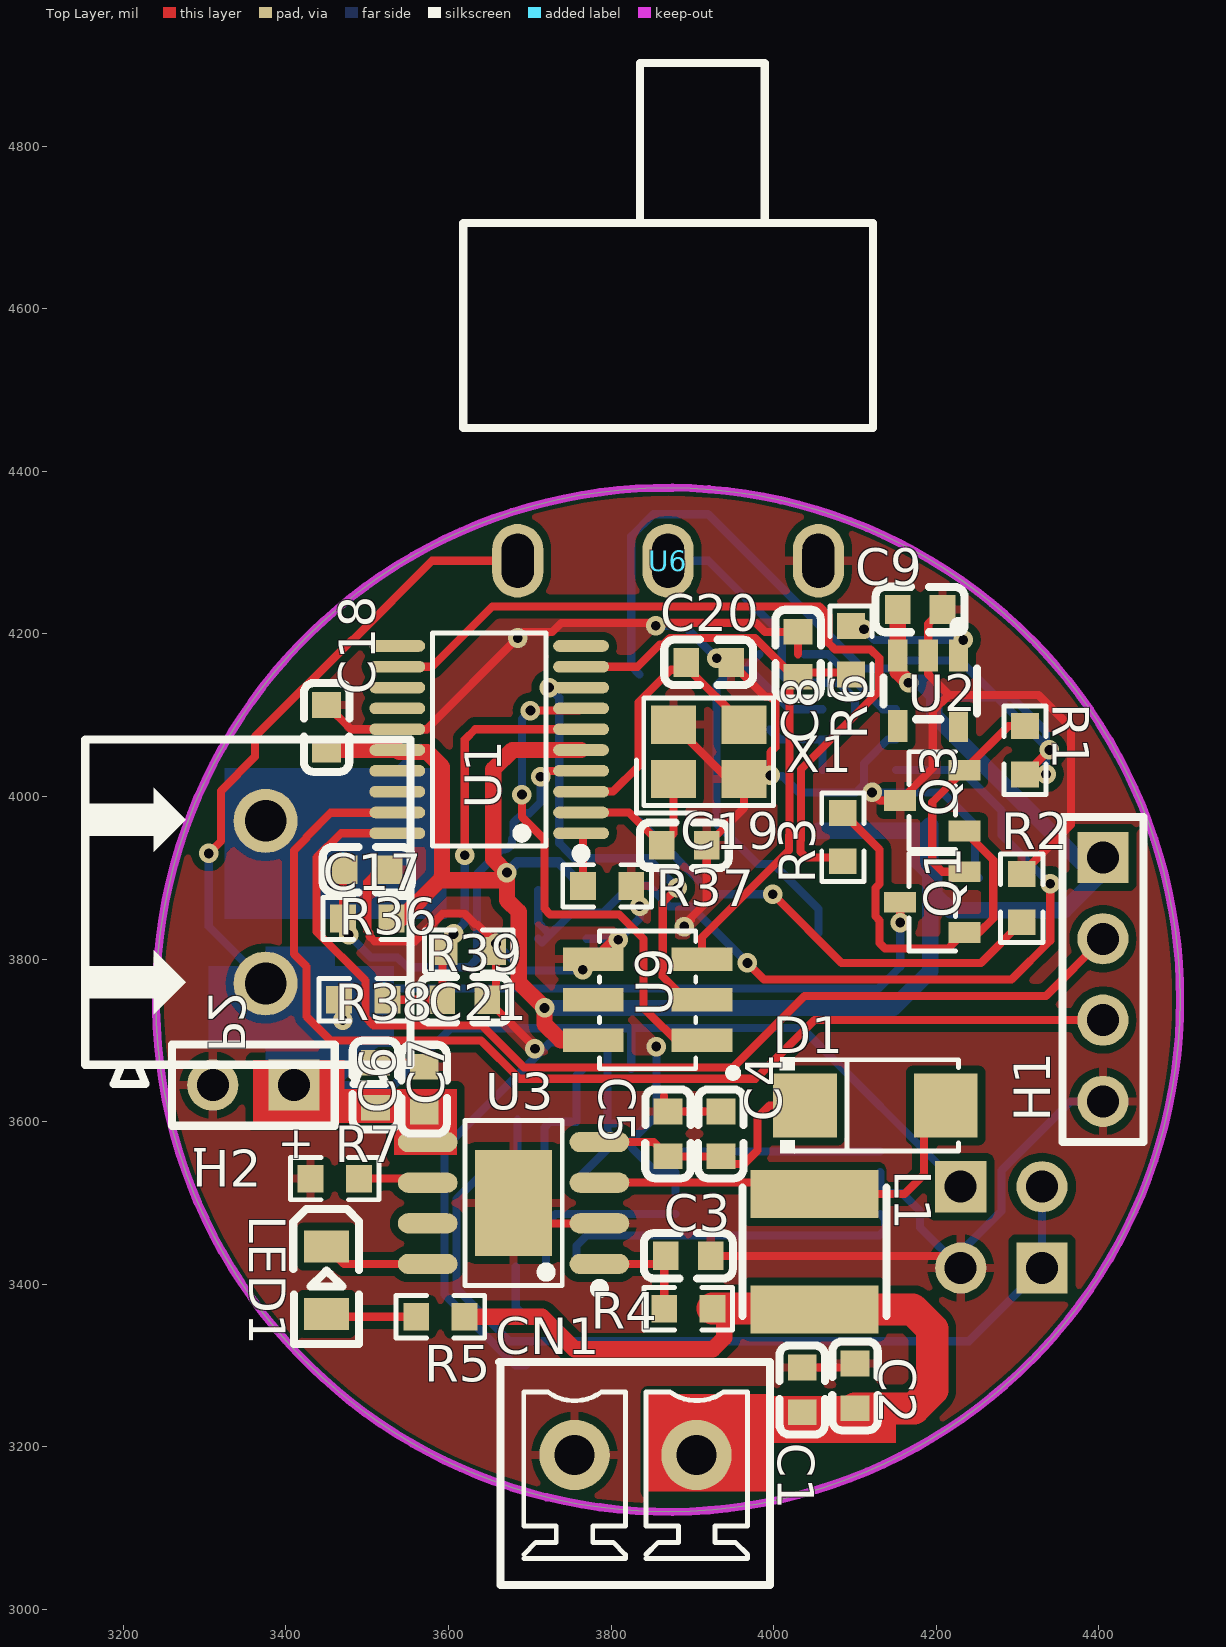
[diagram p0: Top Layer view]
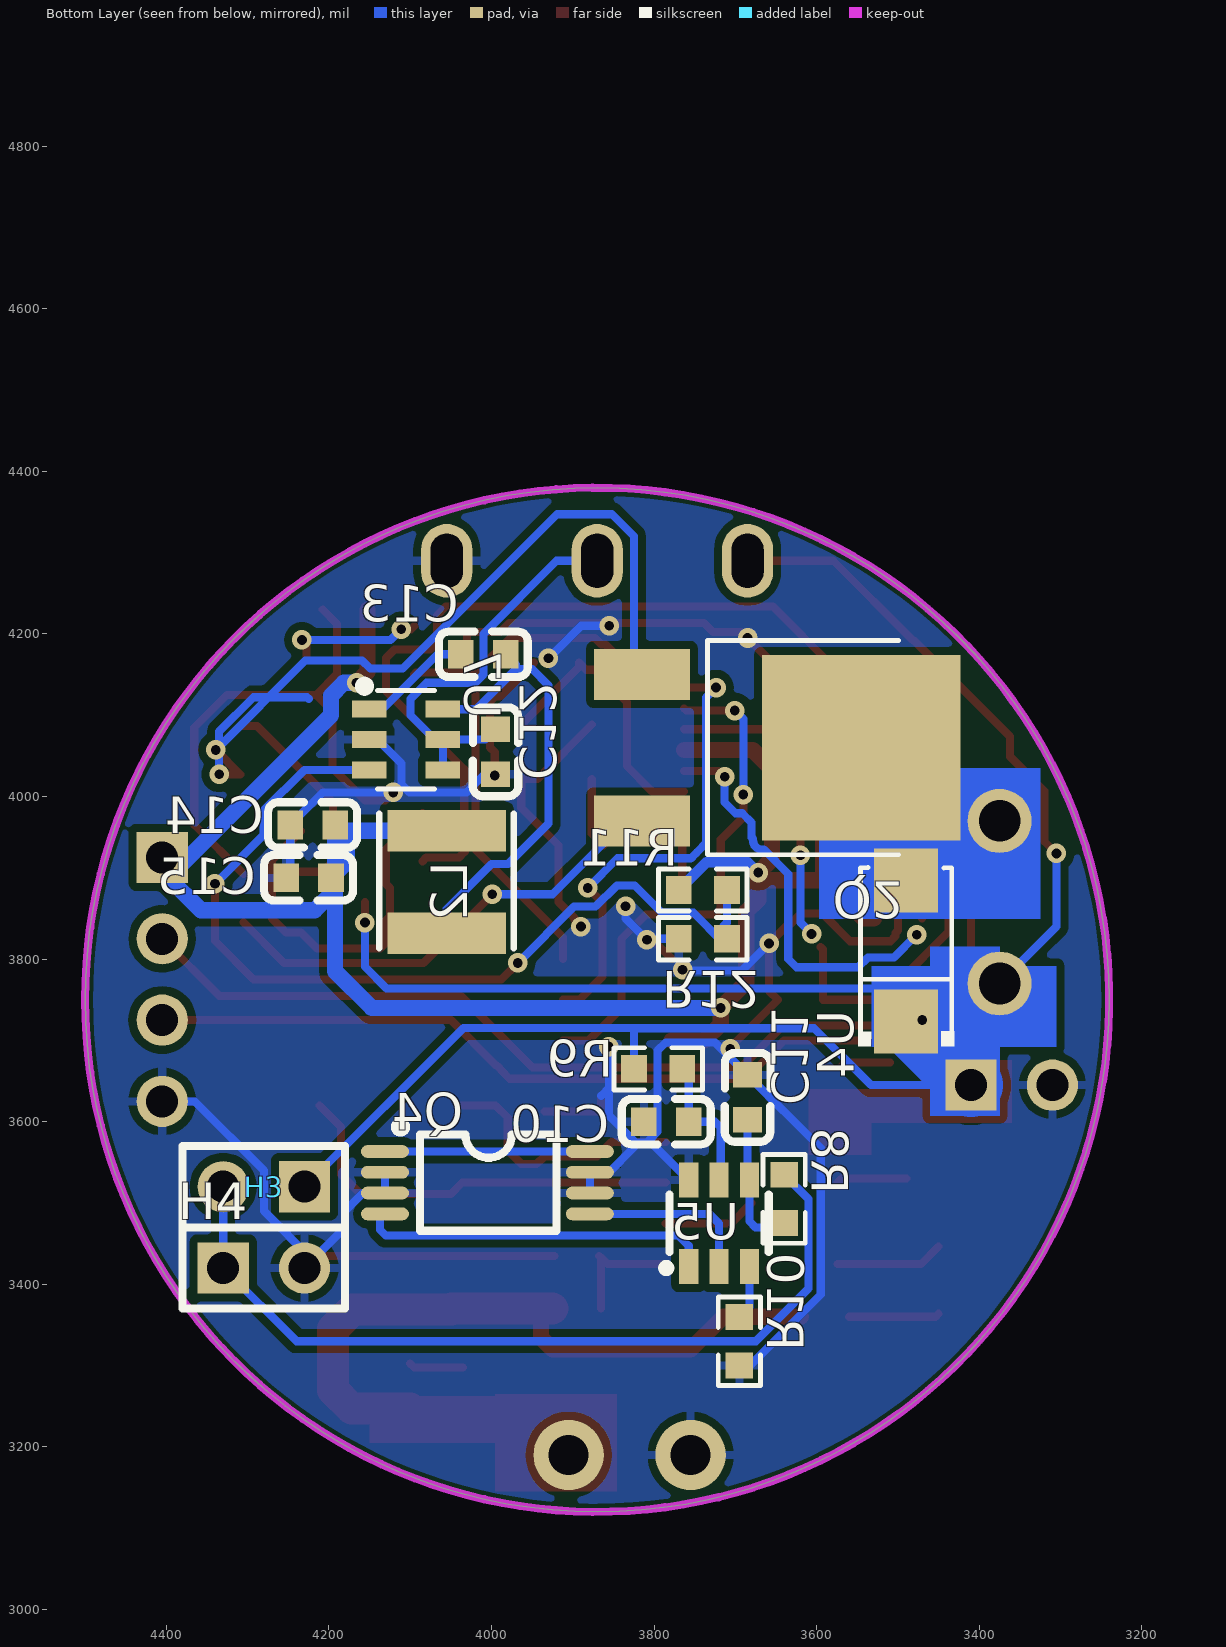
[diagram p1: Bottom Layer view, seen from below]
# Altium PCB MISC80546.pcbdoc
Units mil, origin at the board's own origin, x right, y up, seen from the top; angles counter-clockwise.
Board outline 1259.8 x 1259.8 mil, 2 copper layers (Top Layer, Bottom Layer), stack 62.2 mil thick; 59 components, 40 nets, 172 pads, 33 vias.

## Layer stack, top to bottom
Top Solder Mask Layer: solder mask 0.4, Dk 3.3
Top Layer: signal copper 1.4
Dielectric1: surface 59.4, FR4, Dk 4.5
Bottom Layer: signal copper 1.4
Bottom Solder Mask Layer: solder mask 0.4, Dk 3.3

## Board outline
4499.9,3750 ccw(c3870,3750) 3240.1,3750 ccw(c3870,3750)

## Design rules (kind name [scope] priority, off if disabled: settings)
BoardOutlineClearance copperThickness1oz [All] p0: genericclearance=10 ignorepadtopadclearanceinfootprint=FALSE except(0: Arc-SplitContinuation Track-SplitContinuation SMDPad-SplitContinuation THPad-SplitContinuation Via-SplitContinuation Fill-SplitContinuation Poly-SplitContinuation Region-SplitContinuation Text-SplitContinuation)
BoardOutlineClearance copperThickness2oz [All] p0: genericclearance=10 ignorepadtopadclearanceinfootprint=FALSE except(0: Arc-SplitContinuation Track-SplitContinuation SMDPad-SplitContinuation THPad-SplitContinuation Via-SplitContinuation Fill-SplitContinuation Poly-SplitContinuation Region-SplitContinuation Text-SplitContinuation)
BoardOutlineClearance otherClearance [All] p0: genericclearance=10 ignorepadtopadclearanceinfootprint=FALSE except(0: Arc-SplitContinuation Track-SplitContinuation SMDPad-SplitContinuation THPad-SplitContinuation Via-SplitContinuation Fill-SplitContinuation Poly-SplitContinuation Region-SplitContinuation Text-SplitContinuation)
Clearance copperThickness1oz [All] p1: gap=7 ignorepadtopadclearanceinfootprint=FALSE
Clearance copperThickness2oz [All] p1: gap=7 ignorepadtopadclearanceinfootprint=FALSE
Clearance otherClearance [All] p1: gap=7 ignorepadtopadclearanceinfootprint=FALSE
DiffPairsRouting differentialPair [All] p1: maxuncoupledlength=10 minlimit=6 maxlimit=Infinity mostfreqgap=6 toplayer_minwidth=5 toplayer_prefwidth=10 toplayer_maxwidth=100 bottomlayer_minwidth=5 bottomlayer_prefwidth=10 bottomlayer_maxwidth=100
PasteMaskExpansion pasteMaskExpansion [All] p1: expansion=0
PlaneConnect innerPlane [All] p1: planeconnectstyle=Relief reliefexpansion=20 reliefentries=4 reliefconductorwidth=10 reliefairgap=10
PolygonConnect copperRegion [All] p1: connectstyle=Relief reliefentries=4 reliefconductorwidth=10 polygonreliefangle="90 Angle" airgapwidth=10
RoutingVias viaSize [All] p1: viastyle="Through Hole" holewidth=12.0078 minholewidth=11.811 maxholewidth=248.0314 width=12.0078 minwidth=11.811 maxwidth=248.0314
SolderMaskExpansion solderMaskExpansion [IsVia] p1: useseparateexpansions=TRUE expansion=-1000 expansionbottom=-1000
SolderMaskExpansion solderMaskExpansion [All] p2: useseparateexpansions=TRUE expansion=2 expansionbottom=2
Width copperThickness1oz [All] p1: maxlimit=100 minlimit=5 preferedwidth=10
Width copperThickness2oz [All] p1: maxlimit=100 minlimit=8 preferedwidth=20

## Components (designator, comment, footprint, x,y, rotation, side; value= is the part's Value field where it differs from the comment)
C1 "100nF" C0603 4035,3270 r270 top
C2 "100nF" C0603 4100,3275 r270 top
C3 "100nF" C0603 3895,3435 r180 top
C4 "100nF" C0603 3935,3585 r90 top
C5 "100nF" C0603 3870,3585 r270 top
C6 "100nF" C0603 3510,3645 r90 top
C7 "100nF" C0603 3570,3640 r90 top
C8 "100nF" C0603 4030,4175 r270 top
C9 "100nF" C0603 4180,4230 r0 top
C10 "100nF" C0603 3785,3600 r180 bottom
C11 "100nF" C0603 3685,3630 r90 bottom
C12 "100nF" C0603 3995,4055 r90 bottom
C13 "100nF" C0603 4010,4175 r0 bottom
C14 "100nF" C0603 4220,3965 r180 bottom
C15 "100nF" C0603 4225,3900 r180 bottom
C17 "100nF" C0603 3500,3910 r0 top
C18 "100nF" C0603 3450,4085 r90 top
C19 "100nF" C0603 3890,3940 r0 top
C20 "100nF" C0603 3920,4165 r0 top
C21 "100nF" C0603 3620,3750 r0 top
CN1 "WJ15EDGVC-3.81-02P-14-00A" CONN-TH_WJ15EDGVC-3.81-2P 3830,3190 r0 top
D1 "SS34" SMA_L4.3-W2.6-LS5.2-RD 4125,3620 r0 top
H1 "LAIL-PZ2.54-4P-L" CONN-TH_LAIL-PZ2.54-4P-L 4405,3775 r270 top
H2 "LAIL-PZ2.54-2P-L" CONN-TH_LAIL-PZ2.54-2P-L 3360,3645 r180 top
H3 "LAIL-PZ2.54-2P-L" CONN-TH_LAIL-PZ2.54-2P-L 4280,3520 r0 bottom
H4 "LAIL-PZ2.54-2P-L" CONN-TH_LAIL-PZ2.54-2P-L 4280,3420 r180 bottom
L1 "2.2uH" IND-SMD_L4.0-W4.0_LQH44PN2R2MP0L 4050,3440 r270 top
L2 "4.7uH" IND-SMD_L4.0-W4.0_SMNR4012 4055,3895 r90 bottom
LED1 "KT-0805W" LED0805-R-RD 3450,3405 r270 top
P2 "WJ500V-5.08-2P" CONN-TH_2P-P5.00_WJ500V-5.08-2P 3375,3870 r90 top
Q1 "SS8050(RANGE:200-350)" SOT-23-3_L2.9-W1.3-P1.90-LS2.4-BR 4195,3870 r0 top
Q2 "CMD075N06L" TO-252-2_L6.6-W6.1-P4.57-LS9.9-BR-CW 3680,4060 r0 bottom
Q3 "SS8550 Y2(RANGE:200-350)" SOT-23-3_L2.9-W1.3-P1.90-LS2.4-BR 4195,3995 r0 top
Q4 "AP8205A" TSSOP-8_L4.4-W3.0-P0.65-LS6.4-BL-2 4005,3525 r270 bottom
R1 "10K" R0603 4309.1,4057 r270 top
R2 "10K" R0603 4305,3875 r270 top
R3 "10K" R0603 4085,3950 r90 top
R4 "10K" R0603 3895,3370 r0 top
R5 "10K" R0603 3590,3360 r0 top
R6 "10K" R0603 4095,4180 r90 top
R7 "10K" R0603 3460,3530 r180 top
R8 "10K" R0603 3640,3505 r270 bottom
R9 "10K" R0603 3795,3665 r180 bottom
R10 "10K" R0603 3695,3330 r270 bottom
R11 "10K" R0603 3740,3885 r180 bottom
R12 "10K" R0603 3740,3825 r0 bottom
R36 "10K" R0603 3500,3850 r0 top
R37 "10K" R0603 3795,3890 r0 top
R38 "10K" R0603 3495,3750 r180 top
R39 "10K" R0603 3625,3810 r180 top
U1 "GD32E230F8P6TR" TSSOP-20_L6.5-W4.4-P0.65-LS6.4-BL 3650,4070 r90 top
U2 "SC01T" SOT-23-5_L2.9-W1.6-P0.95-LS2.8-BR 4190,4130 r90 top
U3 "PW4584A" ESOP-8_L4.9-W3.9-P1.27-LS6.0-BL-EP-1 3680,3500 r90 top
U4 "SS36" SMA_L4.3-W2.6-LS5.1-RD 3490,3810 r90 bottom
U5 "HY2120-CB" SOT-23-6_L2.9-W1.6-P0.95-LS2.8-BR 3720,3475 r270 bottom
U6 "SS-12D06G5R" SW-TH_SS-12D06G5R 3870,4290 r180 top
U7 "MT2492" SOT-23-6_L2.9-W1.6-P0.95-LS2.8-BL_3 4105,4070 r270 bottom
U9 "LAIL-PM1.27-3PX2-T" HDR-SMD_6P-P1.27_LAIL-PM1.27-3PX2-T 3845,3750 r90 top locked
X1 "8MHz" CRYSTAL-SMD_4P-L3.2-W2.5-BL 3920,4055 r0 top

## Footprints (in the part's own frame and the unit in brackets; to place one, negate y for a bottom-side part, rotate by r counter-clockwise, add the part's x,y. Pads: shape width x height; smd on the part's side, far side on the other; paste and mask are expansions set on the pad)
C0603 [mil]
  rect 31.5x35.4 smd: 1(-27.6,0) 2(27.6,0)
  silkscreen extent -55,-28 55,28
CONN-TH_2P-P5.00_WJ500V-5.08-2P [mil]
  round 78.7 hole 51.2: 1(-100,0) 2(100,0)
  silkscreen extent -224,-178 200,222
CONN-TH_LAIL-PZ2.54-2P-L [mil]
  rect 63x63 hole 39.4 paste+0 mask+2: 1(-50,0)
  round 63 hole 39.4 paste+0 mask+2: 2(50,0)
  silkscreen extent -100,-50 100,50
CONN-TH_LAIL-PZ2.54-4P-L [mil]
  rect 63x63 hole 39.4 paste+0 mask+2: 1(-150,0)
  round 63 hole 39.4 paste+0 mask+2: 2(-50,0) 3(50,0) 4(150,0)
  silkscreen extent -200,-50 200,50
CONN-TH_WJ15EDGVC-3.81-2P [mil]
  round 86.6 hole 49.2: 1(-75,0) 2(75,0)
  silkscreen extent -168,-160 165,114
CRYSTAL-SMD_4P-L3.2-W2.5-BL [mil]
  rect 55.1x47.2 smd: 1(-43.3,-33.5) 2(43.3,-33.5) 3(43.3,33.5) 4(-43.3,33.5)
  silkscreen extent -89,-75 80,66
ESOP-8_L4.9-W3.9-P1.27-LS6.0-BL-EP-1 [mil]
  oval 24.8x73.4 smd: 1(-75,-105.6) 2(-25,-105.6) 3(25,-105.6) 4(75,-105.6) 5(75,105.6) 6(25,105.6) 7(-25,105.6) 8(-75,105.6)
  rect 129.9x94.5 smd paste+0 mask+2: 9(0,0)
  silkscreen extent -111,-111 101,60
HDR-SMD_6P-P1.27_LAIL-PM1.27-3PX2-T [mil]
  rect 29.1x74.8 smd paste+0 mask+2: 1(-50,-66.9) 2(-50,66.9) 3(0,-66.9) 4(0,66.9) 5(50,-66.9) 6(50,66.9)
  silkscreen extent -95,-110 85,59
IND-SMD_L4.0-W4.0_LQH44PN2R2MP0L [mil]
  rect 59.1x157.5 smd: 1(-70.9,0) 2(70.9,0)
  silkscreen extent -79,-89 79,89
IND-SMD_L4.0-W4.0_SMNR4012 [mil]
  rect 51.2x145.7 smd: 1(-63,0) 2(63,0)
  silkscreen extent -82,-82 84,83
LED0805-R-RD [mil]
  rect 39.4x55.1 smd: 1(41.3,0) 2(-41.3,0)
  silkscreen extent -88,-41 78,40
R0603 [mil]
  rect 31.8x34 smd paste-3937 mask+2: 1(-29.7,0) 2(29.7,0)
  silkscreen extent -55,-26 55,26
SMA_L4.3-W2.6-LS5.1-RD [mil]
  rect 78.7x78.7 smd: 1(-86.6,0) 2(86.6,0)
  silkscreen extent -117,-59 102,59
SMA_L4.3-W2.6-LS5.2-RD [mil]
  rect 78.7x78.7 smd: 1(-86.6,0) 2(86.6,0)
  silkscreen extent -117,-59 102,59
SOT-23-3_L2.9-W1.3-P1.90-LS2.4-BR [mil]
  rect 39.4x25.6 smd: 1(39.4,-37.4) 2(39.4,37.4) 3(-39.4,0)
  silkscreen extent -29,-60 29,60
SOT-23-5_L2.9-W1.6-P0.95-LS2.8-BR [mil]
  rect 39.4x23.6 smd paste+0 mask+2: 1(43.3,-37.4) 2(43.3,0) 3(43.3,37.4) 4(-43.3,37.4) 5(-43.3,-37.4)
  silkscreen extent -35,-60 85,55
SOT-23-6_L2.9-W1.6-P0.95-LS2.8-BL_3 [mil]
  rect 20.9x42.2 smd: 1(-37.4,-45.2) 2(0,-45.2) 3(37.4,-45.2) 4(37.4,45.2) 5(0,45.2) 6(-37.4,45.2)
  silkscreen extent -72,-57 61,35
SOT-23-6_L2.9-W1.6-P0.95-LS2.8-BR [mil]
  rect 43.3x23.6 smd paste+0 mask+2: 1(53.2,-37.4) 2(53.2,0) 3(53.2,37.4) 4(-53.2,37.4) 5(-53.2,0) 6(-53.2,-37.4)
  silkscreen extent -35,-70 60,61
SW-TH_SS-12D06G5R [mil]
  oval 63x90.6 hole 39.4 slot 66.9 at 90 deg: 1(-185,0) 2(0,0) 3(185,0)
  silkscreen extent -252,-612 252,-163
TO-252-2_L6.6-W6.1-P4.57-LS9.9-BR-CW [mil]
  rect 118.1x63 smd: 1(134.8,-90.2) 3(134.8,90.2)
  rect 244.1x228.3 smd: 2(-134.8,0)
  silkscreen extent -180,-132 54,132
TSSOP-8_L4.4-W3.0-P0.65-LS6.4-BL-2 [mil]
  oval 15.7x59.1 smd: 1(-38.4,-126) 2(-12.8,-126) 3(12.8,-126) 4(38.4,-126) 5(38.4,126) 6(12.8,126) 7(-12.8,126) 8(-38.4,126)
  silkscreen extent -74,-113 59,85
TSSOP-20_L6.5-W4.4-P0.65-LS6.4-BL [mil]
  oval 14.3x68.6 smd: 1(-115.2,-113) 2(-89.6,-113) 3(-64,-113) 4(-38.4,-113) 5(-12.8,-113) 6(12.8,-113) 7(38.4,-113) 8(64,-113) 9(89.6,-113) 10(115.2,-113) 11(115.2,113) 12(89.6,113) 13(64,113) 14(38.4,113) 15(12.8,113) 16(-12.8,113) 17(-38.4,113) 18(-64,113) 19(-89.6,113) 20(-115.2,113)
  silkscreen extent -146,-119 131,70

## Via types
v1: diameter 24, hole 12, Top Layer to Bottom Layer, 33 vias

## Nets (pads, with @x,y where several pads share a name; then routed paths per layer and width w, separated by ;. In a path a pad name is that pad's centre, name@x,y a point inside that pad or via, vN(x,y) a via of type N, cw(c..) or ccw(c..) an arc to the next point about the centre after c; other vN are vias at no path point)
$1N2: Q1.1 Q3.1 R3.2 | length 463.1
  Top Layer w10: R3.2 4130,3934.7 4130,3892.4 4125,3887.3 4125,3852.7 4130,3847.6 4130,3820 4137.1,3812.9 4214.7,3812.9 Q1.1 4252.6,3832.6 4270,3850 4270,3922 Q3.1
$1N4: P2.2 Q2.2 U4.2 | length 338.3
  Bottom Layer w10: P2.2 3445,3900 U4.2@3485,3900 ; U4.2 U4.2@3485,3900 ; Q2.2@3565.2,4060 3485,3979.8 U4.2@3485,3900
$1N6: Q2.3 R2.2 | length 563.2
  Top Layer w10: v1(3998.9,3879.8) 4083.4,3795.3 4255,3795.3 R2.2
  Bottom Layer w10: Q2.3@3834.8,3969.8 3924.8,3879.8 v1(3998.9,3879.8)
$1N7: Q2.1 R1.2 | length 1077.5
  Top Layer w10: v1(4335,4027.3) R1.2 v1(4339.1,4057.3)
  Bottom Layer w10: Q2.1@3834.8,4150.2 3824.8,4160.2 3824.8,4320.2 3852,4347.3 3919.1,4347.3 4109.1,4157.3 4149.1,4157.3 4159.1,4167.3 4229.1,4167.3 v1(4339.1,4057.3) ; 4224.8,4120.2 4226.7,4122.1 4292.9,4122.1 4335,4080 v1(4335,4027.3)
$1N8: Q1.2 Q3.2 R1.1 | length 270.6
  Top Layer w10: Q1.2 4207.6,3907.4 4195,3920 4195,3993 Q3.2 4288.6,4086.7 R1.1
$1N16: D1.2 L1.1 U3.3 | length 511.2
  Top Layer w10: U3.3 4035.9,3525 L1.1 4160.9,3510.9 4185,3535 4185,3593.4 D1.2
$1N17: C3.2 R4.1 U3.1 | length 148.8
  Top Layer w10: U3.1 3857.4,3425 C3.2@3865.3,3432.9 ; R4.1 C3.2@3865.3,3432.9 ; C3.2 C3.2@3865.3,3432.9
$1N21: C4.1 C5.2 D1.1 U3.4 | length 317.5
  Top Layer w10: U3.4 3852.4,3575 C5.2 C4.1 3944.5,3547.9 3963.3,3547.9 3980,3564.7 3980,3605 3995,3620 D1.1
$1N23: LED1.1 R5.1 | length 111.8
  Top Layer w10: LED1.1 3453.7,3360 R5.1
$1N25: LED1.2 U3.8 | length 133.2
  Top Layer w10: LED1.2 3471.3,3425 U3.8
$1N26: R7.1 U3.6 | length 86.8
  Top Layer w10: R7.1 3569.4,3530 U3.6
$1N32: R6.2 U2.1 | length 167
  Top Layer w10: R6.2 4099,4205.7 v1(4111,4205.7) ; U2.1 4227.4,4186.8 v1(4233.2,4192.6)
  Bottom Layer w10: v1(4111,4205.7) 4124.1,4192.6 v1(4233.2,4192.6)
$1N42: C10.2 R9.2 U5.5 | length 176.3
  Bottom Layer w10: U5.5 3717.9,3530.2 3717.9,3592.9 3725,3600 C10.2 3757.4,3657.1 R9.2
$1N47: C11.1 R8.2 U5.4 | length 173.7
  Bottom Layer w10: R8.2 3645.3,3470 3675,3470 3682.6,3477.6 U5.4 3685,3530.6 C11.1
$1N55: R10.1 U5.3 | length 67.2
  Bottom Layer w10: U5.3 3682.6,3372.1 R10.1
$1N59: Q4.1 Q4.8 | length 252
  Bottom Layer w10: Q4.8 Q4.1
$1N69: C13.2 U7.1 | length 140.6
  Bottom Layer w10: C13.2 4066.5,4175 4134.1,4107.4 U7.1
$1N70: C13.1 L2.1 U7.6 | length 550.5
  Bottom Layer w10: C13.1 3969.8,4162.3 3969.8,4156.8 ; L2.1 4055,3861.5 3999.8,3916.8 3979.8,3916.8 3929.8,3966.8 3929.8,4136.8 3949.8,4156.8 3969.8,4156.8 ; U7.6 4019.1,4107.4 3969.8,4156.8
$1N198: R37.1 U1.1 | length 65.8
  Top Layer w10: U1.1 3765.3,3952.5 R37.1
+3.3: C9.1 C14.2 C15.2 C18.1 H1.1 L2.2 R11.1 R36.2 U1.5 U1.16 U2.3 U9.2 | length 2692.7
  Top Layer w20: C18.1 3536.7,4057.4 U1.16 3539.4,4054.8 3573.7,4054.8 3592,4036.4 3592,3899.9 3589.1,3897 ; R36.2 3542.1,3850 3589.1,3897 ; U1.5 3678.6,4057.2 3655,4033.6 3655,3923.2 v1(3671.8,3906.4) ; U9.2 3738.1,3700 3718.1,3720 v1(3718.1,3740) 3686.5,3771.6 3686.5,3858.1 3671.8,3872.8 v1(3671.8,3906.4) ; C9.1@4152.6,4229.8 U2.3 4152.6,4153.3 v1(4165.9,4140) ; 3589.1,3897 3662.4,3897 v1(3671.8,3906.4)
  Bottom Layer w13.2: v1(3671.8,3906.4) 3684.6,3919.2 3735.4,3919.2 R11.1
  Bottom Layer w20: v1(3718.1,3740) 4147.4,3740 4192.4,3785 C15.2@4192.4,3905 ; L2.2 C14.2@4177.8,3958 ; v1(4165.9,4140) 4181.7,4140 4197.4,4124.2 4197.4,4100 H1.1@4397.4,3900 ; H1.1 4397.4,3917.4 H1.1@4397.4,3900 ; C14.2@4177.8,3958 4177.8,3919.6 C15.2@4192.4,3905 ; C14.2@4177.8,3958 4185.4,3958 C14.2 C15.2@4192.4,3905 ; C15.2@4192.4,3905 C15.2 4197.4,3880 4217.4,3860 4357.4,3860 H1.1@4397.4,3900
+5V: C1.2 C2.2 CN1.2 L1.2 R4.2 R5.2 | length 843.7
  Top Layer w20: R5.2 3715,3360 3755,3320 3925,3320 3939.1,3334.1 3939.1,3355.5 R4.2
  Top Layer w39.4: R4.2 4049.1,3370 L1.2 4170.9,3369.1 4195,3345 4195,3270 4172.4,3247.4 C2.2
ADC: C21.1 R38.1 R39.2 U1.6 | length 526.9
  Top Layer w10: R38.1 C21.1 3592.4,3812.1 R39.2@3595.3,3815 ; v1(3620,3927.8) 3620,4070 3632.8,4082.8 U1.6
  Bottom Layer w10: v1(3606.2,3831) 3620,3844.8 v1(3620,3927.8)
BAT1-: H3.2 H4.1 R8.1 | length 1036.5
  Bottom Layer w10: R8.1 3610,3504.7 3610,3394.7 3674.7,3330 4240,3330 H4.1 H3.2
CO: Q4.5 U5.2 | length 217
  Bottom Layer w10: U5.2 3720,3475 3731.6,3486.6 Q4.5
DO: Q4.4 U5.1 | length 435.5
  Bottom Layer w10: U5.1 3757.4,3447.4 3770,3460 4130,3460 4137.1,3467.1 4137.1,3480.5 Q4.4
FB: R11.2 R12.1 U7.3 | length 1118.4
  Top Layer w10: v1(3967.6,3795.3) 3988,3775 4292.6,3775 4340.2,3822.6 v1(4340.2,3892.6)
  Bottom Layer w10: R12.1 3715,3820.3 3751.7,3857 3790.1,3857 3823.8,3890.7 3845.8,3890.7 3872,3864.6 3898.4,3864.6 v1(3967.6,3795.3) ; R11.2 3710.3,3844.8 R12.1@3720.2,3834.9 ; U7.3 4230.2,4032.6 4280.2,3982.6 4280.2,3952.6 v1(4340.2,3892.6)
GND: C1.1 C2.1 C3.1 C4.2 C5.1 C6.2 C7.2 C8.1 C9.2 C10.1 C11.2 C12.1 C14.1 C15.1 C17.2 C18.2 C19.2 C20.2 C21.2 CN1.1 H1.4 H2.2 H4.2 Q3.3 Q4.2 Q4.3 Q4.6 Q4.7 R2.1 R7.2 R10.2 R12.2 R37.2 R39.1 U1.15 U2.2 U3.2 U3.9 U5.6 U6.1 U7.2 U9.6 X1.2 X1.4 | length 5236.4
  Top Layer w10: C18.2 3479.8,4082.8 U1.15 3572.8,4082.8 v1(3685,4195) 3692.6,4202.6 3727.6,4202.6 3738.7,4213.6 3978.1,4213.6 3989.2,4202.6 C8.1 4030,4175 ; C6.2 3565,3672.6 C7.2 ; C17.2 3515,3910 3500,3895 3500,3835 3502.8,3832.2 3502.8,3828.4 3509.2,3822 3558.9,3822 3592.9,3856 3619.5,3856 3633,3842.5 3635.3,3842.5 v1(3658.5,3819.3) 3658.5,3761 C21.2 3706.3,3691.3 v1(3706.3,3689.8) v1@3706.3,3688.4 ; U3.9 3705,3475 U3.2 ; U9.6 3801.8,3823.7 v1(3808.7,3823.7) ; 3865,3631.9 3865,3617.6 C5.1 C4.2 ; X1.4 3943.6,4021.5 X1.2 3963.3,3985.8 C19.2 3917.6,3870.4 3897.9,3850.7 3897.9,3847.9 v1(3890,3840) ; C3.1 4215,3435 H4.2 ; C20.2 3989.5,4123.1 3995.4,4123.1 4001.9,4116.6 4001.9,4060.3 3996,4054.5 v1(3996,4025.9) ; C1.1 4095,3297.6 C2.1 ; v1(4120.9,4005) 4130.9,3995 Q3.3 4195.6,4035 4195.6,4105 4215.6,4125 ; C9.2 4190,4212.4 U2.2 4190,4150.6 4215.6,4125 ; R2.1 4365.6,3965.3 4365.6,4085 4325.6,4125 4215.6,4125
  Bottom Layer w10: v1(3658.5,3819.3) 3691.9,3786 v1@3765,3786 ; R10.2 3682.2,3300.3 3595,3387.6 3595,3567.6 C11.2 3725,3697.6 3785.6,3697.6 3795.6,3687.6 3795.6,3597.6 ; U5.6 3805.6,3576.4 3805.6,3577.6 ; R12.2 3807.5,3825 v1(3808.7,3823.7) 3835,3850 v1(3835,3865) ; C10.1 3810.1,3597.6 3795.6,3597.6 ; 3825.6,3577.6 3825.6,3567.6 3855.6,3537.6 Q4.7@3878.8,3537.6 ; v1(3855,4210) 3890,4210 v1(3930,4170) ; v1(3855.6,3692.4) 3855.6,3641.3 ; 3865,3631.9 3855.6,3641.3 ; Q4.6 Q4.7 ; C12.1 C12.1@3997.4,4025 ; C12.1@4000.9,4025 4010.9,4025 4030.9,4005 4100.9,4005 4110.9,4015 ; Q4.2 Q4.3 4157.8,3512.2 4180,3490 4180,3470 H4.2 ; U7.2 4140.2,4070 4110.9,4040.7 4110.9,4015 ; H4.2@4220,3430 4280,3490 4280,3540 4365,3625 H1.4 ; C15.1 4247.6,3905 C14.1 4207.6,4005 v1(4120.9,4005) 4110.9,4015 ; 3795.6,3597.6 3795.6,3587.6 3805.6,3577.6 ; 3805.6,3577.6 3808.6,3574.6 3822.7,3574.6 3855.6,3607.6 3855.6,3641.3
  other v1: 3765,3787
KEY: C8.2 R6.1 U1.9 U9.5 | length 762.2
  Top Layer w10: U1.9 3832.3,4159.6 3859.8,4187 3864.5,4187 3872.5,4195 3976.9,4195 C8.2@4019.5,4152.4 ; U9.5 3911.9,3826.9 4018.9,3933.9 4018.9,3951.9 4019.5,3952.4 C8.2@4019.5,4152.4 ; R6.1 4092.9,4152.4 C8.2@4019.5,4152.4
MCU_KEY: U2.5
NRST: C17.1 R36.1 U1.4 | length 564.6
  Top Layer w10: R36.1 3470.3,3907.9 C17.1 ; v1@3712.4,4031.6 3712.4,4025 v1(3713.2,4024.2) 3720.5,4031.6 U1.4
  Bottom Layer w10: v1(3477,3830) 3504.8,3802.2 3537,3802.2 3549.3,3790 3625,3790 3635,3800 3635,3904.8 3665,3934.8 3667.2,3934.8 ccw(c3667.2,3945.8) 3678.2,3945.8 3678.2,3948.1 3680,3949.8 3680,3967.9 3691.5,3979.4 3699.7,3979.4 3713.2,3992.9 v1(3713.2,4024.2)
OSIN: C19.1 U1.2 X1.1 | length 203.6
  Top Layer w10: U1.2 3822,3980.4 C19.1 3876.7,3954.3 X1.1
OSOUT: C20.1 U1.3 X1.3 | length 347.3
  Top Layer w10: U1.3 3802.3,4006 3833.5,4037.2 3833.5,4116 3873.5,4156 3883.5,4156 C20.1 3892.4,4159.3 X1.3
PA6: R3.1 U1.12 | length 1004.8
  Top Layer w10: U1.12 3579.6,4159.6 3653.7,4233.7 4056.2,4233.7 4067,4222.9 4067,4189.2 4075.4,4180.9 4119.1,4180.9 4129.8,4170.2 4129.8,4129.8 4033.5,4033.5 4033.5,3946.6 4032.9,3946.1 4032.9,3932.1 4040,3925 4080.3,3925 R3.1
SCL: U1.7 U9.1 | length 633.8
  Top Layer w10: v1(3690.2,4002.4) 3690.2,3974.9 3717.9,3947.1 3717.9,3862.1 3725,3855 3810,3855 3840,3825 3840,3740 3864.6,3715.4 3865.1,3715.4 3880.5,3700 U9.1 ; v1(3700.7,4105.8) 3760.4,4105.8 U1.7
  Bottom Layer w10: v1(3690.2,4002.4) 3690.2,4095.2 v1(3700.7,4105.8)
SDA: U1.8 U9.3 | length 580.8
  Top Layer w10: v1(3723.7,4134) U1.8 ; v1(3881.5,3887.5) 3863.5,3869.6 3863.5,3778.4 3891.9,3750 U9.3
  Bottom Layer w10: v1(3723.7,4134) 3736.1,4121.6 3736.1,3942.6 3746.9,3931.9 ; 3746.81,3931.82 ccw(c3755.7,3938.3) 3749.22,3929.41 ; 3749.3,3929.5 3754.8,3924 3845.1,3924 v1(3881.5,3887.5)
SWCLK: H1.2 U1.20 | length 1331.3
  Top Layer w10: U1.20 3467.7,3954.8 3437.7,3924.8 3437.7,3833.7 3497.7,3773.7 3497.7,3728.5 3507.7,3718.5 3641.3,3718.5 3693,3666.8 3949.7,3666.8 4037.7,3754.8 4334.8,3754.8 H1.2
SWDIO: H1.3 U1.19 | length 1399
  Top Layer w10: U1.19 3536.5,3980 3455,3980 3425.4,3950.4 3425.4,3949.1 3410,3933.8 3410,3806.2 3425.4,3790.9 3425.4,3729.6 3455,3700 3640,3700 3687.2,3652.8 3977.8,3652.8 3989.1,3664.1 ; 3989.08,3664.15 cw(c3999,3659.4) 3994.25,3669.32 ; 3994.3,3669.3 4050,3725 H1.3
vbat: C6.1 C7.1 H2.1 H3.1 P2.1 Q1.3 R9.1 R38.2 U3.5 U4.1 U6.3 | length 313.4
  Top Layer w10: R38.2 3470,3745.3 v1(3470,3725) ; v1(4155.6,3845) Q1.3
  Bottom Layer w10: 3533.1,3645 3603.1,3715 ; R9.1 3824.7,3715
  Bottom Layer w78.7: H2.1 3488.4,3723.4 U4.1
VBAT:  | length 2555.7
  Top Layer w10: v1(3305,3930) 3320,3945 3320,4006.9 3362.1,4049 3362.1,4073.7 3481.1,4192.7 3482.3,4192.7 3579.6,4290 3685,4290
  Bottom Layer w10: v1(3305,3930) 3305,3840 3375,3770 3443.4,3770 3449.4,3764 ; 3410,3645 3533.1,3645 ; 3490,3723.4 3449.4,3764 ; 3603.1,3715 3824.7,3715 ; 3824.7,3665 3824.7,3714.7 3825.4,3715.4 4034.6,3715.4 4230,3520 ; 4155.6,3845 4155.6,3790.6 4129,3764 3449.4,3764
VBAT_K: C12.2 U6.2 U7.4 U7.5 | length 509.4
  Bottom Layer w10: U6.2 3919.8,4290 4009.8,4200 4009.8,4150 4019.8,4140 4079.8,4140 4099.8,4120 4099.8,4100 4069.8,4070 U7.5 ; C12.2 4007.6,4070 U7.5 ; U7.4 U7.5
pads on no net: U1.10 U1.11 U1.13 U1.14 U1.17 U1.18 U2.4 U3.7 U9.4

## Polygon pours and split planes (outlines as drawn)
GND on Bottom Layer (solid, remove dead copper, pour order 2): 3015,4520 3015,3000 4550,3000 4550,4520
GND on Top Layer (solid, remove dead copper, pour order 0): 3000,4420 3000,3065 4580,3065 4580,4420

## Keep-outs
Board Outline Layer:
  lines w10: 3240.2,3738.8 3241,3716.5 3242.6,3694.2 3244.9,3671.9 3248.1,3649.8 3252,3627.8 3256.8,3605.9 3262.3,3584.3 3268.5,3562.8 3275.6,3541.6 3283.3,3520.6 3291.8,3499.9 3301.1,3479.6 3311,3459.5 3321.7,3439.9 3333,3420.6 3345.1,3401.8 3357.8,3383.4 3371.1,3365.4 3385.1,3348 3399.6,3331 3414.8,3314.6 3430.5,3298.7 3446.8,3283.4 3463.7,3268.7 3481,3254.5 3498.8,3241 3517.1,3228.2 3535.9,3216 3555,3204.5 3574.6,3193.6 3594.5,3183.5 3614.8,3174.1 3635.4,3165.4 3656.3,3157.4 3677.5,3150.2 3698.9,3143.8 3720.5,3138.1 3742.3,3133.2 3764.3,3129 3786.4,3125.7 3808.6,3123.1 3830.9,3121.3 3853.2,3120.3 3875.6,3120.1 3897.9,3120.7 3920.3,3122.1 3942.5,3124.3 3964.7,3127.2 3986.7,3131 4008.6,3135.5 4030.3,3140.8 4051.9,3146.9 4073.1,3153.7 4094.2,3161.3 4114.9,3169.6 4135.4,3178.7 4155.5,3188.5 4175.2,3199 4194.6,3210.1 4213.5,3222 4232.1,3234.5 4250.1,3247.7 4267.7,3261.5 4284.8,3275.9 4301.4,3291 4317.4,3306.6 4332.8,3322.7 4347.7,3339.4 4362,3356.6 4375.6,3374.3 4388.7,3392.5 4401,3411.2 4412.7,3430.2 4423.7,3449.7 4434,3469.5 4443.6,3489.7 4452.5,3510.2 4460.6,3531.1 4468,3552.2 4474.7,3573.5 4480.6,3595.1 4485.7,3616.8 4490,3638.8 4493.6,3660.9 4496.4,3683 4498.3,3705.3 4499.5,3727.6 4499.9,3750 4499.5,3772.4 4498.3,3794.7 4496.4,3817 4493.6,3839.1 4490,3861.2 4485.7,3883.2 4480.6,3904.9 4474.7,3926.5 4468,3947.8 4460.6,3968.9 4452.5,3989.8 4443.6,4010.3 4434,4030.5 4423.7,4050.3 4412.7,4069.8 4401,4088.8 4388.7,4107.5 4375.6,4125.7 4362,4143.4 4347.7,4160.6 4332.8,4177.3 4317.4,4193.4 4301.4,4209 4284.8,4224.1 4267.7,4238.5 4250.1,4252.3 4232.1,4265.5 4213.5,4278 4194.6,4289.9 4175.2,4301 4155.5,4311.5 4135.4,4321.3 4114.9,4330.4 4094.2,4338.7 4073.1,4346.3 4051.9,4353.1 4030.3,4359.2 4008.6,4364.5 3986.7,4369 3964.7,4372.8 3942.5,4375.7 3920.3,4377.9 3897.9,4379.3 3875.6,4379.9 3853.2,4379.7 3830.9,4378.7 3808.6,4376.9 3786.4,4374.3 3764.3,4371 3742.3,4366.8 3720.5,4361.9 3698.9,4356.2 3677.5,4349.8 3656.3,4342.6 3635.4,4334.6 3614.8,4325.9 3594.5,4316.5 3574.6,4306.4 3555,4295.5 3535.9,4284 3517.1,4271.8 3498.8,4259 3481,4245.5 3463.7,4231.3 3446.8,4216.6 3430.5,4201.3 3414.8,4185.4 3399.6,4169 3385.1,4152 3371.1,4134.6 3357.8,4116.6 3345.1,4098.2 3333,4079.4 3321.7,4060.1 3311,4040.5 3301.1,4020.4 3291.8,4000.1 3283.3,3979.4 3275.6,3958.4 3268.5,3937.2 3262.3,3915.7 3256.8,3894.1 3252,3872.2 3248.1,3850.2 3244.9,3828.1 3242.6,3805.8 3241,3783.5 3240.2,3761.2 3240.2,3738.8

## Other copper
Top Layer:
  region net +5V: 3984.6,3262.3 3984.6,3205 4150,3205 4150,3262.3
  region net +5V: 3845.9,3264.9 3845.9,3145.6 3995.4,3145.6 3995.4,3264.9
  region net VBAT: 3460,3640 3460,3598.9 3610,3598.9 3610,3640
  region net VBAT: 3532.9,3640 3532.9,3559.5 3610,3559.5 3610,3640
  region net VBAT: 3360,3675.4 3360,3598.9 3471.9,3598.9 3471.9,3675.4
Bottom Layer:
  region net $1N4: 3325,4035 3325,3849.7 3596.9,3849.7 3596.9,4035
  region net VBAT: 3305,3791.3 3305,3692.5 3532.5,3692.5 3532.5,3791.3
  region net VBAT: 3375,3815 3375,3607.6 3460,3607.6 3460,3815

## Silkscreen, mask and mechanical layers (free items; w line width, h text height)
Top Silkscreen Layer:
  text "+" at 3390,3555 h39.4
  text "-" at 3285,3550 h39.4